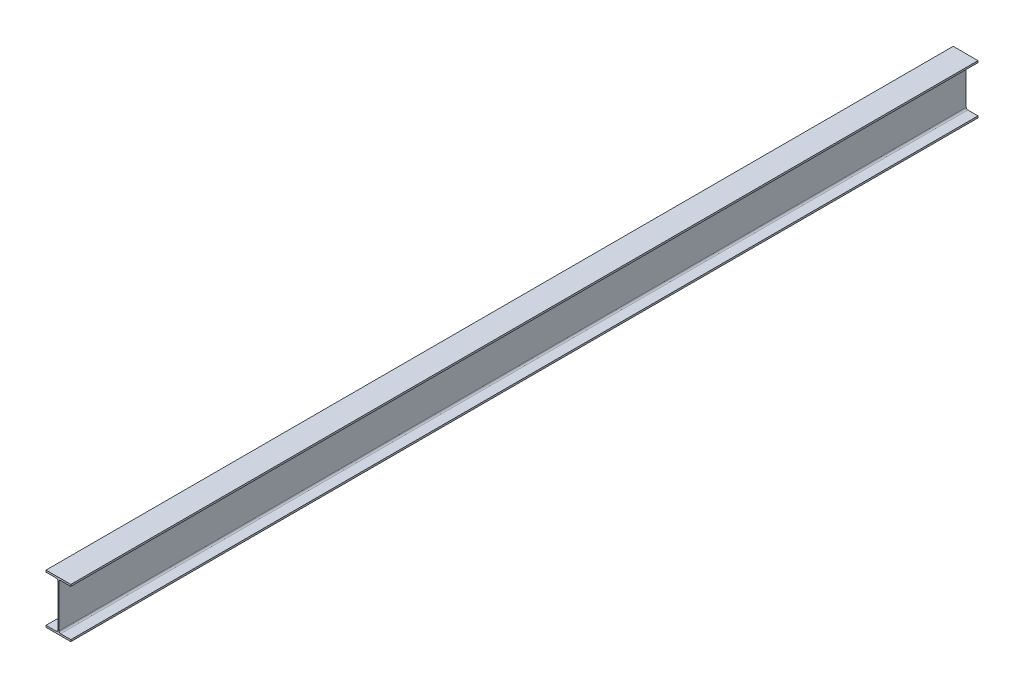
SolidWorks part; units mm, degrees
ref_plane "Front Plane" through (0, 0, 0) normal (0, 0, 1) x (1, 0, 0)
ref_plane "Top Plane" through (0, 0, 0) normal (0, 1, 0) x (1, 0, 0)
ref_plane "Right Plane" through (0, 0, 0) normal (1, 0, 0) x (0, 0, -1)
other "Configuration Table"
sketch "Sketch1" plane through (0, 0, 0) normal (0, 0, 1) x (1, 0, 0)
  line L0 (0, 0) -> (0, 250) construction
  line L1 (62.5, 0) -> (-62.5, 0)
  line L2 (-62.5, 0) -> (-62.5, 9)
  line L3 (-62.5, 9) -> (-11, 9)
  line L4 (3, 17) -> (3, 233)
  line L6 (-62.5, 241) -> (-62.5, 250)
  line L7 (-62.5, 250) -> (62.5, 250)
  line L8 (-3, 17) -> (-3, 233)
  line L9 (62.5, 241) -> (62.5, 250)
  line L10 (11, 241) -> (62.5, 241)
  line L11 (62.5, 9) -> (11, 9)
  line L12 (62.5, 0) -> (62.5, 9)
  line L13 (-11, 241) -> (-62.5, 241)
  arc A0 (11, 9) -> (3, 17) centre (11, 17) cw
  arc A1 (-3, 17) -> (-11, 9) centre (-11, 17) cw
  arc A2 (3, 233) -> (11, 241) centre (11, 233) cw
  arc A3 (-3, 233) -> (-11, 241) centre (-11, 233) ccw
  point P18 (3, 9)
  point P21 (-3, 9)
  point P24 (3, 241)
  point P27 (-3, 241)
  dimension "D6" = 8
  dimension "D1" = 250
  dimension "D2" = 125
  dimension "D3" = 6
  dimension "D4" = 9
  dimension "D5" = 9
extrude "Boss-Extrude1" add sketch "Sketch1" along normal blind 4570
